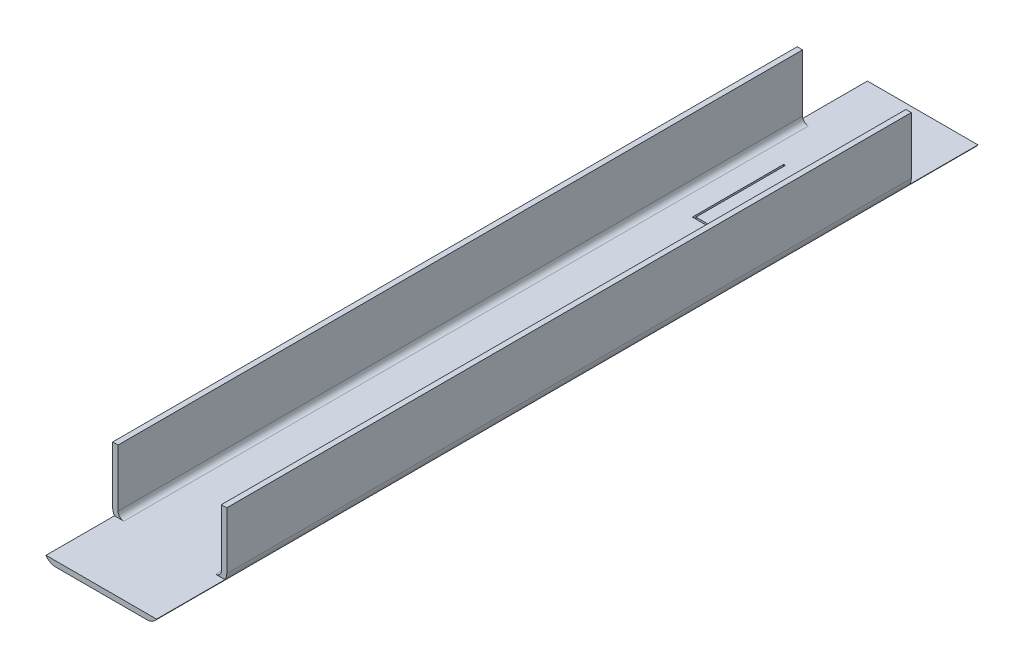
from build123d import *

# Parameters (mm, degrees)
BOSS_EXTRUDE1_DEPTH = 228.6
SKETCH2_W           = 19.05
SKETCH2_H           = 17.55
CUT_EXTRUDE1_DEPTH  = 232.579198116
CUT_EXTRUDE2_DEPTH  = 232.579198116


with BuildPart() as part:
    # Sketch1 → Boss-Extrude1 (new body)
    with BuildSketch(Plane.XY):
        with BuildLine():
            Line((30.25, 3.1), (30.25, 19.05))
            Line((30.25, 19.05), (31.75, 19.05))
            Line((31.75, 19.05), (31.75, 3.2))
            ThreePointArc((31.75, 3.2), (30.8127417, 0.9372583), (28.55, 0))
            Line((28.55, 0), (3.2, 0))
            ThreePointArc((3.2, 0), (0.9372583, 0.9372583), (0, 3.2))
            Line((0, 3.2), (0, 19.05))
            Line((0, 19.05), (1.5, 19.05))
            Line((1.5, 19.05), (1.5, 3.1))
            ThreePointArc((1.5, 3.1), (1.96862915, 1.96862915), (3.1, 1.5))
            Line((3.1, 1.5), (28.65, 1.5))
            ThreePointArc((28.65, 1.5), (29.78137085, 1.96862915), (30.25, 3.1))
        make_face()
    extrude(amount=BOSS_EXTRUDE1_DEPTH)

    # Sketch2 → Cut-Extrude1 (cut, through all)
    with BuildSketch(Plane(origin=(0, 0, 0), x_dir=(0, 0, -1), z_dir=(1, 0, 0))):
        with Locations((-9.525, 10.275)):
            Rectangle(SKETCH2_W, SKETCH2_H)
        with Locations((-219.075, 10.275)):
            Rectangle(SKETCH2_W, SKETCH2_H)
    extrude(amount=CUT_EXTRUDE1_DEPTH, mode=Mode.SUBTRACT)

    # Sketch3 → Cut-Extrude2 (cut, through all)
    with BuildSketch(Plane(origin=(0, 0, 0), x_dir=(1, 0, 0), z_dir=(0, 1, 0))):
        Polygon((22.821846385, -57.15), (8.928153615, -57.15), (8.928153615, -31.75), (9.428153615, -31.75), (9.428153615, -56.65), (22.321846385, -56.65), (22.321846385, -31.75), (22.821846385, -31.75), align=None)
    extrude(amount=CUT_EXTRUDE2_DEPTH, mode=Mode.SUBTRACT)


solid = part.part
